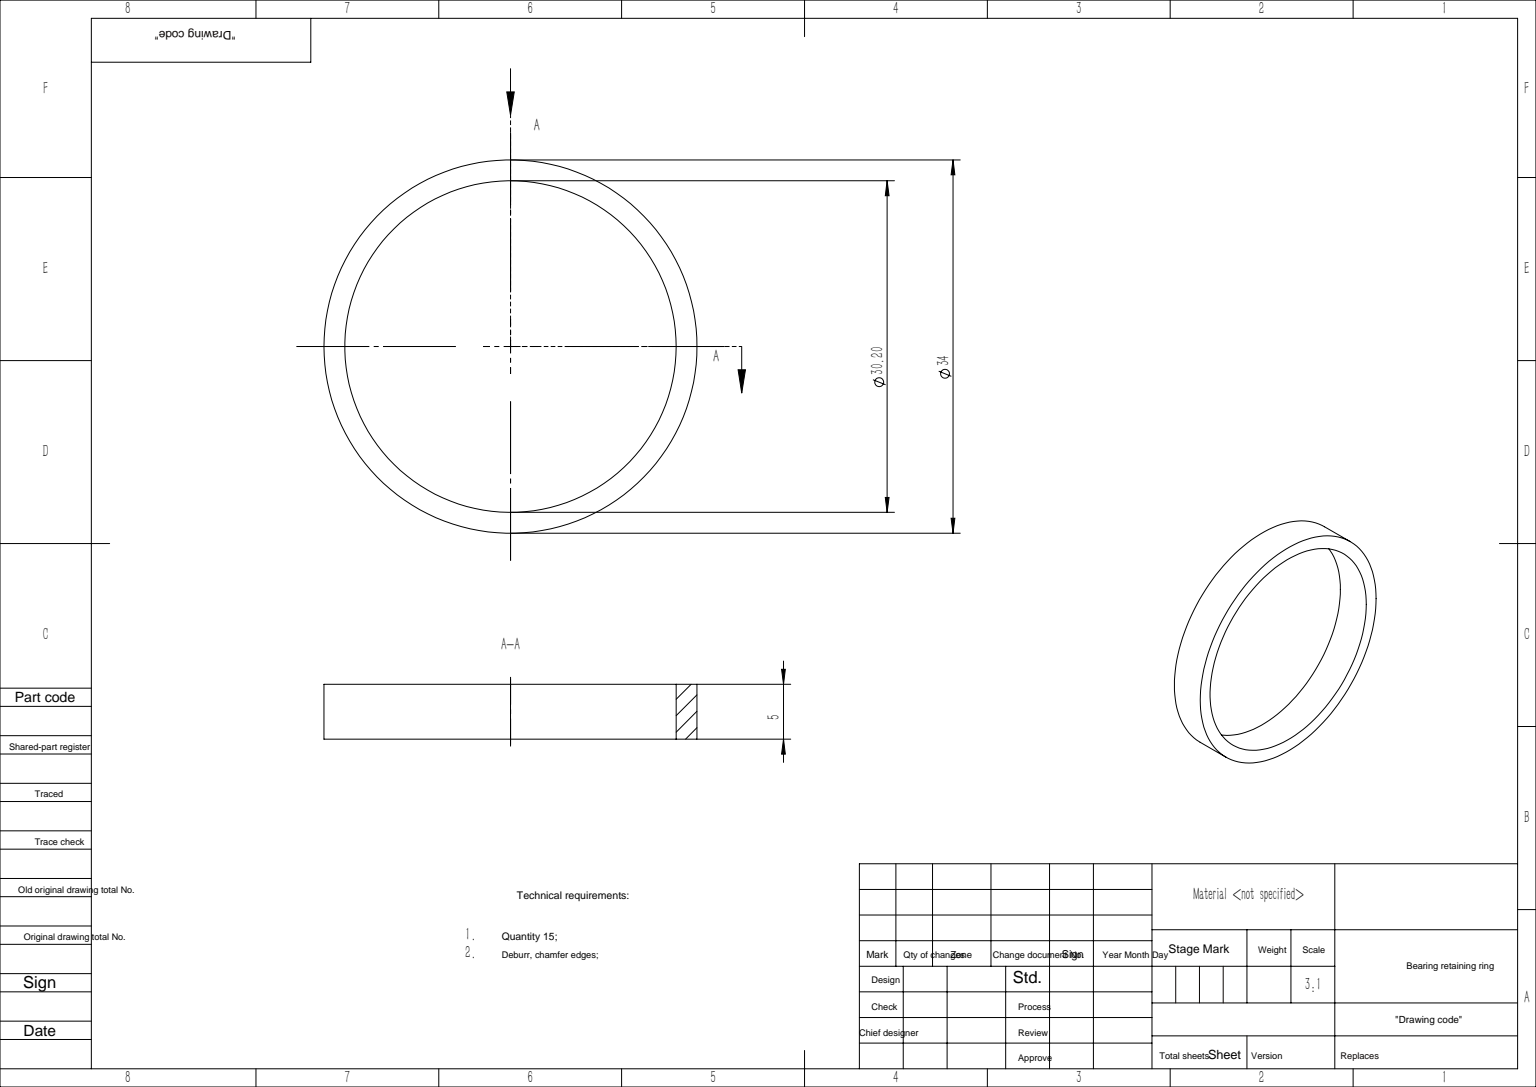
from build123d import *

# Parameters (mm, degrees)
SKETCH_1_R      = 17
SKETCH_1_R_2    = 15.1
EXTRUDE_1_DEPTH = 5


with BuildPart() as part:
    # 草图1 → 凸台-拉伸1 (new body)
    with BuildSketch(Plane(origin=(0, 0, 0), x_dir=(0, 0, -1), z_dir=(1, 0, 0))):
        Circle(SKETCH_1_R)
        Circle(SKETCH_1_R_2, mode=Mode.SUBTRACT)
    extrude(amount=EXTRUDE_1_DEPTH)


solid = part.part
